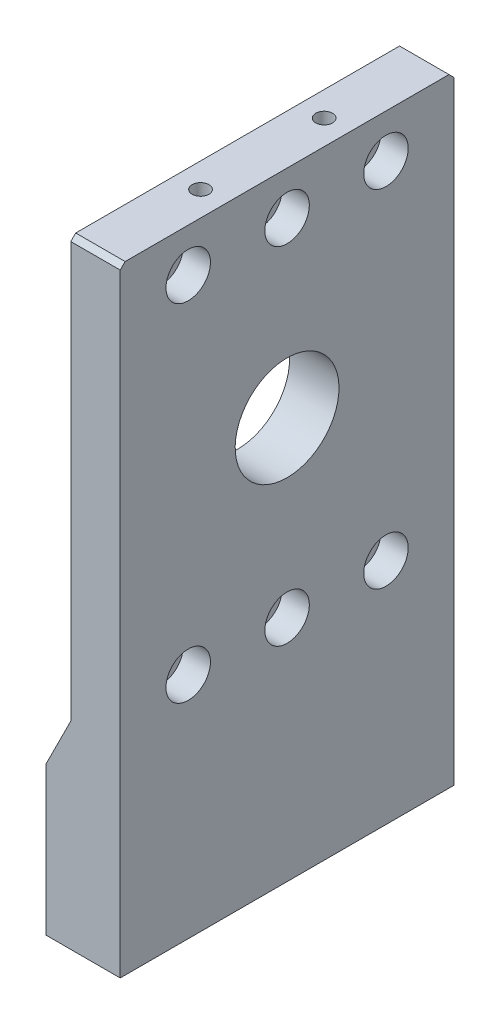
SolidWorks part; units mm, degrees
ref_plane "Front Plane" through (0, 0, 0) normal (0, 0, 1) x (1, 0, 0)
ref_plane "Top Plane" through (0, 0, 0) normal (0, 1, 0) x (1, 0, 0)
ref_plane "Right Plane" through (0, 0, 0) normal (1, 0, 0) x (0, 0, -1)
sketch "Sketch1" plane through (0, 0, 0) normal (0, 0, 1) x (1, 0, 0)
  line L0 (0, 0) -> (0, 60)
  line L1 (0, 60) -> (10, 80)
  line L2 (10, 80) -> (10, 250)
  line L3 (10, 250) -> (30, 250)
  line L4 (30, 250) -> (30, 0)
  line L5 (30, 0) -> (0, 0)
  dimension "D1" = 30
  dimension "D2" = 20
  dimension "D3" = 60
  dimension "D4" = 250
  dimension "D5" = 20
extrude "Boss-Extrude1" add sketch "Sketch1" along normal mid plane 135
hole_wizard "M8 Tapped Hole1" positions "Sketch3" profile "Sketch2" tap size "M8" standard "GB"
sketch "Sketch3" plane through (0, 0, 0) normal (0, -1, 0) x (1, 0, 0)
  line L0 (15, 67.5) -> (15, -51.8972) construction
  line L1 (0, 67.5) -> (30, 67.5) construction
  line L3 (0, 0) -> (48, 0) construction
  point P1 (6, -42.5)
  point P3 (24, -42.5)
  point P5 (24, 0)
  point P7 (6, 0)
  point P9 (6, 42.5)
  point P11 (24, 42.5)
  dimension "D1" = 18
  dimension "D2" = 85
sketch "Sketch2" plane through (6, 0, -42.5) normal (1, 0, 0) x (0, 0, -1)
  line L0 (0, 0) -> (0, 21.7929)
  line L1 (0, 21.7929) -> (3.4, 19.75)
  line L2 (3.4, 19.75) -> (3.4, 0)
  line L5 (3.4, 0) -> (0, 0)
  line L10 (0, 21.7929) -> (-3.4, 19.75) construction
  line L11 (0, -6.35) -> (0, 107.95) construction
  dimension "螺纹孔钻头直径" = 6.8
  dimension "螺纹孔钻头深度" = 19.75
  dimension "导头角度" = 118
cosmetic thread "Cosmetic Thread1" parameters "D1"=16, "D2"=8
cosmetic thread "Cosmetic Thread2" parameters "D1"=16, "D2"=8
cosmetic thread "Cosmetic Thread3" parameters "D1"=16, "D2"=8
cosmetic thread "Cosmetic Thread4" parameters "D1"=16, "D2"=8
cosmetic thread "Cosmetic Thread5" parameters "D1"=16, "D2"=8
cosmetic thread "Cosmetic Thread6" parameters "D1"=16, "D2"=8
hole_wizard "Hole size per socket head cap screw type1" positions "Sketch7" profile "Sketch6" counterbore size "M10" standard "Gb" end condition through all
sketch "Sketch7" plane through (30, 0, 0) normal (1, 0, 0) x (0, 0, -1)
  line L0 (0, 250) -> (0, -12.5931) construction
  line L1 (-67.5, 250) -> (67.5, 250) construction
  point P2 (-40, 232.5)
  point P4 (40, 232.5)
  point P6 (40, 92.5)
  point P8 (-40, 92.5)
  point P18 (0, 232.5)
  point P20 (0, 92.5)
  dimension "D1" = 80
  dimension "D2" = 17.5
  dimension "D3" = 140
sketch "Sketch6" plane through (30, 232.5, 40) normal (0, 1, 0) x (0, 0, -1)
  line L0 (0, 0) -> (0, 30)
  line L1 (0, 30) -> (5.5, 30)
  line L3 (5.5, 30) -> (5.5, 11)
  line L4 (5.5, 11) -> (9, 11)
  line L5 (9, 11) -> (9, 0)
  line L7 (9, 0) -> (0, 0)
  line L11 (0, -6.35) -> (0, 107.95) construction
  dimension "通孔孔直径" = 11
  dimension "通孔孔深度" = 30
  dimension "柱形沉头孔直径" = 18
  dimension "柱形沉头孔深度" = 11
sketch "Sketch8" plane through (10, 0, 0) normal (-1, 0, 0) x (0, 0, 1)
  line L0 (67.5, 250) -> (-67.5, 250) construction
  line L1 (0, 250) -> (0, 80) construction
  line L2 (67.5, 80) -> (-67.5, 80) construction
  circle A0 centre (0, 162.5) radius 21
  dimension "D1" = 42
  dimension "D2" = 87.5
extrude "Cut-Extrude1" cut sketch "Sketch8" against normal through all
hole_wizard "M8 Tapped Hole2" positions "Sketch10" profile "Sketch9" tap size "M8" standard "GB"
sketch "Sketch10" plane through (0, 250, 0) normal (0, 1, 0) x (-1, 0, 0)
  line L0 (-20, -67.5) -> (-20, 72.0244) construction
  line L1 (-30, -67.5) -> (-10, -67.5) construction
  line L3 (-10, 0) -> (-30, 0) construction
  line L4 (-10, 67.5) -> (-10, -67.5) construction
  line L5 (-30, 67.5) -> (-30, -67.5) construction
  point P0 (-20, -25)
  point P3 (-20, 25)
  dimension "D1" = 50
sketch "Sketch9" plane through (20, 250, -25) normal (1, 0, 0) x (0, 0, 1)
  line L0 (0, 0) -> (0, 21.7929)
  line L1 (0, 21.7929) -> (3.4, 19.75)
  line L2 (3.4, 19.75) -> (3.4, 0)
  line L5 (3.4, 0) -> (0, 0)
  line L10 (0, 21.7929) -> (-3.4, 19.75) construction
  line L11 (0, -6.35) -> (0, 107.95) construction
  dimension "螺纹孔钻头直径" = 6.8
  dimension "螺纹孔钻头深度" = 19.75
  dimension "导头角度" = 118
cosmetic thread "Cosmetic Thread7" parameters "D1"=16, "D2"=8
cosmetic thread "Cosmetic Thread8" parameters "D1"=16, "D2"=8
chamfer "Chamfer1" distance 2 angle 45 2 edges at (20, 250, -67.5) (20, 250, 67.5)
hole_wizard "M3 Tapped Hole1" positions "Sketch12" profile "Sketch11" tap size "M3" standard "Gb"
sketch "Sketch12" plane through (10, 0, 0) normal (-1, 0, 0) x (0, 0, 1)
  line L2 (-67.5, 248) -> (-67.5, 80) construction
  line L3 (65.5, 250) -> (-65.5, 250) construction
  point P1 (-37.5, 152.5)
  point P4 (-37.5, 172.5)
  dimension "D1" = 30
  dimension "D2" = 20
  dimension "D3" = 77.5
sketch "Sketch11" plane through (10, 152.5, -37.5) normal (0, 1, 0) x (0, 0, 1)
  line L0 (0, 0) -> (0, 8.2511)
  line L1 (0, 8.2511) -> (1.25, 7.5)
  line L2 (1.25, 7.5) -> (1.25, 0)
  line L5 (1.25, 0) -> (0, 0)
  line L10 (0, 8.2511) -> (-1.25, 7.5) construction
  line L11 (0, -6.35) -> (0, 107.95) construction
  dimension "螺纹孔钻头直径" = 2.5
  dimension "螺纹孔钻头深度" = 7.5
  dimension "导头角度" = 118
cosmetic thread "Cosmetic Thread9" parameters "D1"=6, "D2"=3
cosmetic thread "Cosmetic Thread10" parameters "D1"=6, "D2"=3
